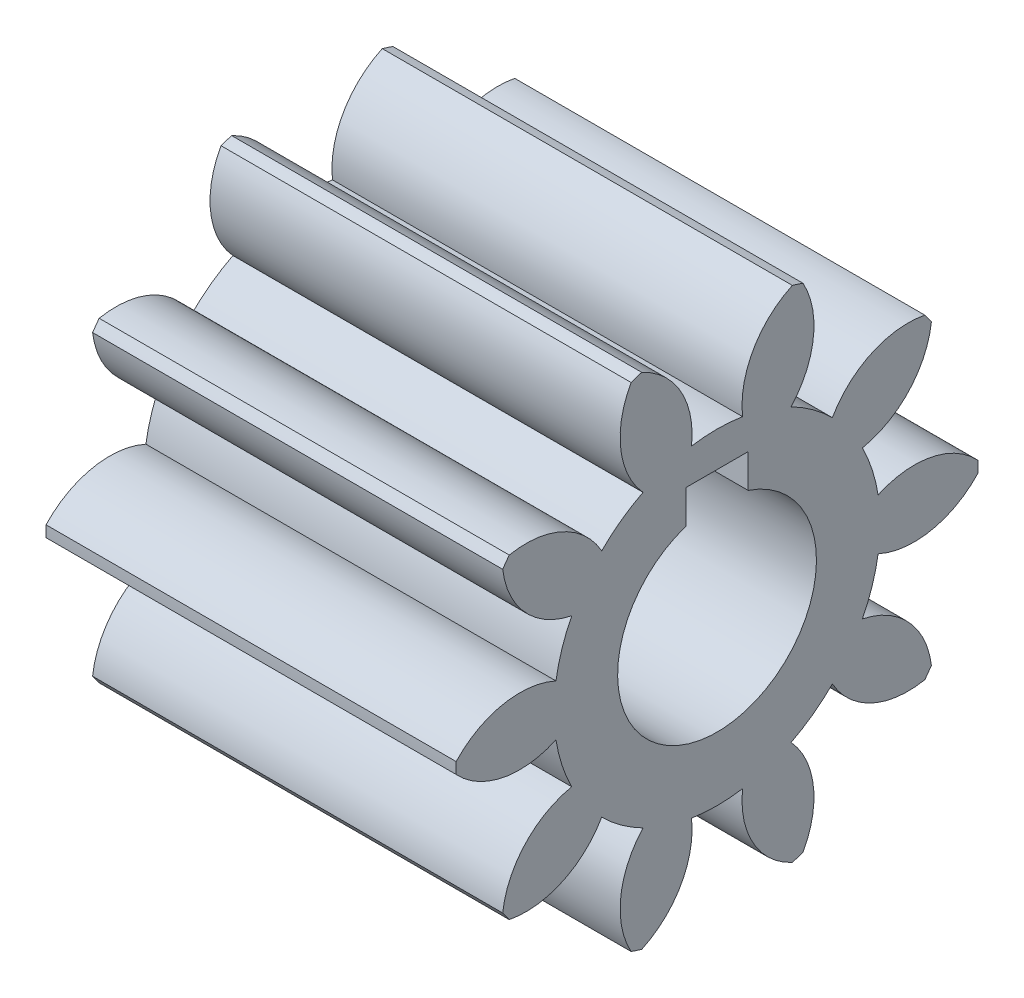
SolidWorks part; units mm, degrees
ref_plane "Front Plane" through (0, 0, 0) normal (0, 0, 1) x (1, 0, 0)
ref_plane "Top Plane" through (0, 0, 0) normal (0, 1, 0) x (1, 0, 0)
ref_plane "Right Plane" through (0, 0, 0) normal (1, 0, 0) x (0, 0, -1)
other "Configuration Table"
ref_plane "Plane1" through (33, 0, 0) normal (1, 0, 0) x (0, 0, -1)
sketch "Sketch1" plane through (33, 0, 0) normal (1, 0, 0) x (0, 0, -1)
  line L0 (2.5, 10.3) -> (2.5, 7.5993)
  line L1 (-2.5, 7.5993) -> (-2.5, 10.3)
  line L2 (-2.5, 10.3) -> (2.5, 10.3)
  arc A0 (20.9952, 0.4501) -> (12.9625, 2.0526) centre (15.8682, -4.3158) ccw
  arc A1 (12.9625, 2.0526) -> (11.6934, 5.9586) centre (0, 0) ccw
  arc A2 (11.6934, 5.9586) -> (17.25, 11.9765) centre (10.3008, 12.8187) ccw
  arc A3 (17.25, 11.9765) -> (16.7209, 12.7048) centre (0, 0) ccw
  arc A4 (16.7209, 12.7048) -> (9.2804, 9.2797) centre (15.3744, 5.8355) ccw
  arc A5 (9.2804, 9.2797) -> (5.9578, 11.6938) centre (0, 0) ccw
  arc A6 (5.9578, 11.6938) -> (6.9159, 19.8285) centre (0.7989, 16.4252) ccw
  arc A7 (6.9159, 19.8285) -> (6.0598, 20.1067) centre (0, 0) ccw
  arc A8 (6.0598, 20.1067) -> (2.0535, 12.9624) centre (9.0081, 13.7579) ccw
  arc A9 (2.0535, 12.9624) -> (-2.0535, 12.9624) centre (0, 0) ccw
  arc A10 (-2.0535, 12.9624) -> (-6.0598, 20.1067) centre (-9.0081, 13.7579) ccw
  arc A11 (-6.0598, 20.1067) -> (-6.9159, 19.8285) centre (0, 0) ccw
  arc A12 (-6.9159, 19.8285) -> (-5.9578, 11.6938) centre (-0.7989, 16.4252) ccw
  arc A13 (-5.9578, 11.6938) -> (-9.2804, 9.2797) centre (0, 0) ccw
  arc A14 (-9.2804, 9.2797) -> (-16.7209, 12.7048) centre (-15.3744, 5.8355) ccw
  arc A15 (-16.7209, 12.7048) -> (-17.25, 11.9765) centre (0, 0) ccw
  arc A16 (-17.25, 11.9765) -> (-11.6934, 5.9586) centre (-10.3008, 12.8187) ccw
  arc A17 (-11.6934, 5.9586) -> (-12.9625, 2.0526) centre (0, 0) ccw
  arc A18 (-12.9625, 2.0526) -> (-20.9952, 0.4501) centre (-15.8682, -4.3158) ccw
  arc A19 (-20.9952, 0.4501) -> (-20.9952, -0.4501) centre (0, 0) ccw
  arc A20 (-20.9952, -0.4501) -> (-12.9625, -2.0526) centre (-15.8682, 4.3158) ccw
  arc A21 (-12.9625, -2.0526) -> (-11.6934, -5.9586) centre (0, 0) ccw
  arc A22 (-11.6934, -5.9586) -> (-17.25, -11.9765) centre (-10.3008, -12.8187) ccw
  arc A23 (-17.25, -11.9765) -> (-16.7209, -12.7048) centre (0, 0) ccw
  arc A24 (-16.7209, -12.7048) -> (-9.2804, -9.2797) centre (-15.3744, -5.8355) ccw
  arc A25 (-9.2804, -9.2797) -> (-5.9578, -11.6938) centre (0, 0) ccw
  arc A26 (-5.9578, -11.6938) -> (-6.9159, -19.8285) centre (-0.7989, -16.4252) ccw
  arc A27 (-6.9159, -19.8285) -> (-6.0598, -20.1067) centre (0, 0) ccw
  arc A28 (-6.0598, -20.1067) -> (-2.0535, -12.9624) centre (-9.0081, -13.7579) ccw
  arc A29 (-2.0535, -12.9624) -> (2.0535, -12.9624) centre (0, 0) ccw
  arc A30 (2.0535, -12.9624) -> (6.0598, -20.1067) centre (9.0081, -13.7579) ccw
  arc A31 (6.0598, -20.1067) -> (6.9159, -19.8285) centre (0, 0) ccw
  arc A32 (6.9159, -19.8285) -> (5.9578, -11.6938) centre (0.7989, -16.4252) ccw
  arc A33 (5.9578, -11.6938) -> (9.2804, -9.2797) centre (0, 0) ccw
  arc A34 (9.2804, -9.2797) -> (16.7209, -12.7048) centre (15.3744, -5.8355) ccw
  arc A35 (16.7209, -12.7048) -> (17.25, -11.9765) centre (0, 0) ccw
  arc A36 (17.25, -11.9765) -> (11.6934, -5.9586) centre (10.3008, -12.8187) ccw
  arc A37 (11.6934, -5.9586) -> (12.9625, -2.0526) centre (0, 0) ccw
  arc A38 (12.9625, -2.0526) -> (20.9952, -0.4501) centre (15.8682, 4.3158) ccw
  arc A39 (20.9952, -0.4501) -> (20.9952, 0.4501) centre (0, 0) ccw
  arc A40 (2.5, 7.5993) -> (-2.5, 7.5993) centre (0, 0) cw
extrude "Boss-Extrude1" add sketch "Sketch1" against normal blind 33
